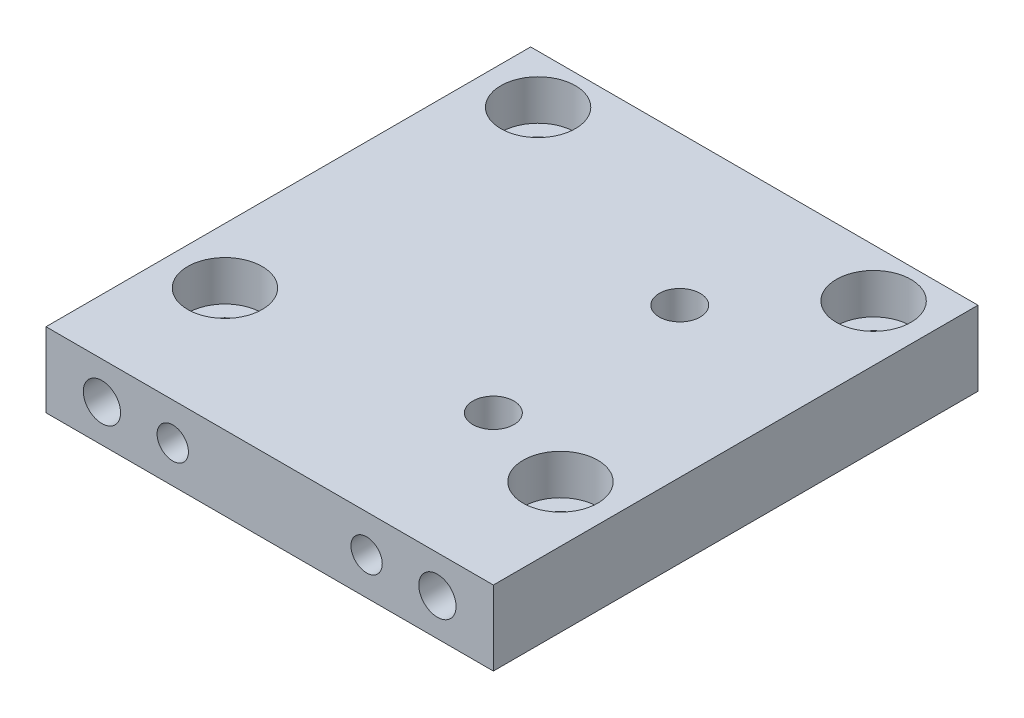
from build123d import *

# Parameters (mm, degrees)
SKETCH_1_W                   = 60
SKETCH_1_H                   = 65
EXTRUDE_1_DEPTH              = 5
HOLE_WIZARD_M5_1_D           = 5.5
HOLE_WIZARD_M5_1_CBORE_D     = 10
HOLE_WIZARD_M5_1_CBORE_DEPTH = 5.4
F_5_0MM_1_D                  = 5
F_5_0MM_1_DEPTH              = 7
HOLE_WIZARD_M5_1_2_D         = 4.2
HOLE_WIZARD_M5_1_2_DEPTH     = 12.4
HOLE_WIZARD_M5_1_2_TIP       = 1.2618073
HOLE_WIZARD_M5_2_D           = 5.5
HOLE_WIZARD_M5_2_CBORE_D     = 10
HOLE_WIZARD_M5_2_CBORE_DEPTH = 5.4


with BuildPart() as part:
    # 草图1 → 凸台-拉伸1 (new, symmetric)
    with BuildSketch(Plane(origin=(0, 0, 0), x_dir=(1, 0, 0), z_dir=(0, 1, 0))):
        Rectangle(SKETCH_1_W, SKETCH_1_H)
    extrude(amount=EXTRUDE_1_DEPTH, both=True)

    # Hole Wizard M5 _1 (through all)
    with Locations(Plane(origin=(0, 5, 0), x_dir=(1, 0, 0), z_dir=(0, 1, 0))):
        with Locations((-22.5, 26), (-22.5, -16), (22.5, -16), (22.5, 26)):
            CounterBoreHole(HOLE_WIZARD_M5_1_D / 2, HOLE_WIZARD_M5_1_CBORE_D / 2, HOLE_WIZARD_M5_1_CBORE_DEPTH)

    # Ø5.0mm 暗销孔1
    with Locations(Plane.XY.offset(32.5)):
        with Locations((-22.5, 0), (22.5, 0)):
            Hole(F_5_0MM_1_D / 2, depth=F_5_0MM_1_DEPTH)

    # Hole Wizard M5 _1 2
    with Locations(Plane.XY.offset(32.5)):
        with Locations((-13, 0), (13, 0)):
            Hole(HOLE_WIZARD_M5_1_2_D / 2, depth=HOLE_WIZARD_M5_1_2_DEPTH)
            with Locations((0, 0, -(HOLE_WIZARD_M5_1_2_DEPTH + HOLE_WIZARD_M5_1_2_TIP / 2))):  # 118° drill point
                Cone(0, HOLE_WIZARD_M5_1_2_D / 2, HOLE_WIZARD_M5_1_2_TIP, mode=Mode.SUBTRACT)

    # M5 六角凹头螺钉的柱形沉头孔2 (through all)
    with Locations(Plane(origin=(0, -5, 0), x_dir=(-1, 0, 0), z_dir=(0, -1, 0))):
        with Locations((-10, -12.5), (-10, 12.5)):
            CounterBoreHole(HOLE_WIZARD_M5_2_D / 2, HOLE_WIZARD_M5_2_CBORE_D / 2, HOLE_WIZARD_M5_2_CBORE_DEPTH)


solid = part.part
